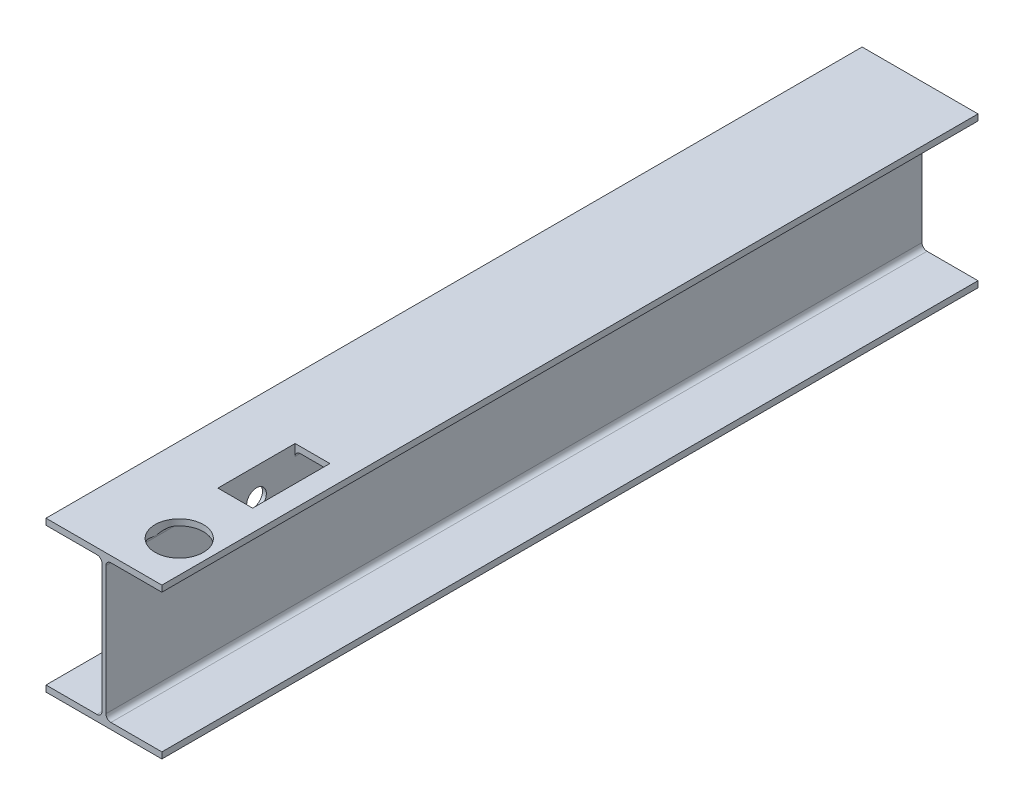
SolidWorks part; units mm, degrees
material "Q235"
ref_plane "Front Plane" through (0, 0, 0) normal (0, 0, 1) x (1, 0, 0)
ref_plane "Top Plane" through (0, 0, 0) normal (0, 1, 0) x (1, 0, 0)
ref_plane "Right Plane" through (0, 0, 0) normal (1, 0, 0) x (0, 0, -1)
sketch "Sketch1" plane through (0, 0, 0) normal (0, 0, 1) x (1, 0, 0)
  line L0 (0, 0) -> (300, 0)
  line L1 (300, 0) -> (300, 16)
  line L2 (300, 16) -> (168, 16)
  line L3 (155, 29) -> (155, 361)
  line L4 (168, 374) -> (300, 374)
  line L5 (300, 374) -> (300, 390)
  line L6 (300, 390) -> (0, 390)
  line L7 (0, 390) -> (0, 374)
  line L8 (0, 374) -> (132, 374)
  line L9 (145, 361) -> (145, 29)
  line L10 (132, 16) -> (0, 16)
  line L11 (0, 16) -> (0, 0)
  line L12 (150, 390) -> (150, 0) construction
  arc A0 (168, 16) -> (155, 29) centre (168, 29) cw
  arc A1 (145, 29) -> (132, 16) centre (132, 29) cw
  arc A2 (155, 361) -> (168, 374) centre (168, 361) cw
  arc A3 (132, 374) -> (145, 361) centre (132, 361) cw
  point P21 (155, 374)
  dimension "D7" = 13
  dimension "D1" = 390
  dimension "D2" = 300
  dimension "D3" = 10
  dimension "D4" = 5
  dimension "D5" = 16
  dimension "D6" = 16
extrude "Boss-Extrude1" add sketch "Sketch1" along normal blind 2113
sketch "Sketch2" plane through (0, 390, 0) normal (0, 1, 0) x (1, 0, 0)
  line L0 (300, -2113) -> (300, 0) construction
  line L1 (245, -1623) -> (155, -1623)
  line L2 (245, -1623) -> (245, -1823)
  line L3 (245, -1823) -> (155, -1823)
  line L4 (155, -1623) -> (155, -1823)
  line L5 (300, -2113) -> (0, -2113) construction
  circle A0 centre (218, -1986) radius 62.5
  dimension "D1" = 125
  dimension "D2" = 82
  dimension "D3" = 127
  dimension "D4" = 200
  dimension "D5" = 90
  dimension "D6" = 163
  dimension "D7" = 55
extrude "Cut-Extrude1" cut sketch "Sketch2" against normal blind 30
sketch "Sketch3" plane through (155, 0, 0) normal (1, 0, 0) x (0, 0, -1)
  line L0 (-2113, 29) -> (-2113, 361) construction
  line L1 (-1623, 390) -> (-1823, 390) construction
  circle A0 centre (-1723, 315) radius 25.5
  dimension "D1" = 51
  dimension "D2" = 390
  dimension "D3" = 75
extrude "Cut-Extrude2" cut sketch "Sketch3" against normal up to next
